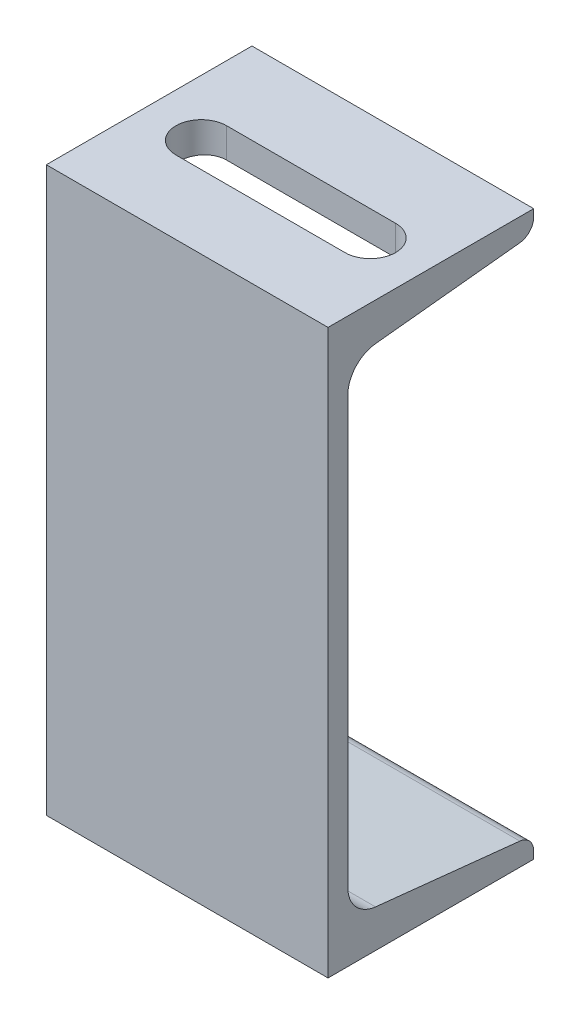
from build123d import *

# Parameters (mm, degrees)
C_20A_1_DEPTH       = 100
CUT_EXTRUDE_1_DEPTH = 16


with BuildPart() as part:
    # Sketch1 → C 槽 20A(1) (new body)
    with BuildSketch(Plane(origin=(0, 0, 0), x_dir=(0, 0, -1), z_dir=(1, 0, 0))):
        with BuildLine():
            Line((73, 200), (0, 200))
            Line((0, 200), (0, 0))
            Line((0, 0), (73, 0))
            Line((73, 0), (73, 2.579337993))
            ThreePointArc((73, 2.579337993), (71.58729654, 6.259556328), (68.074906548, 8.049208417))
            Line((68.074906548, 8.049208417), (16.850186904, 13.433143402))
            ThreePointArc((16.850186904, 13.433143402), (9.82540692, 17.012447581), (7, 24.372884251))
            Line((7, 24.372884251), (7, 175.627115749))
            ThreePointArc((7, 175.627115749), (9.82540692, 182.987552419), (16.850186904, 186.566856598))
            Line((16.850186904, 186.566856598), (68.074906548, 191.950791583))
            ThreePointArc((68.074906548, 191.950791583), (71.58729654, 193.740443672), (73, 197.420662007))
            Line((73, 197.420662007), (73, 200))
        make_face()
    extrude(amount=C_20A_1_DEPTH)

    # 草图2 → 切除-拉伸1 (cut)
    with BuildSketch(Plane(origin=(0, 200, 0), x_dir=(1, 0, 0), z_dir=(0, 1, 0))):
        with BuildLine():
            Line((20, 44), (80, 44))
            ThreePointArc((80, 44), (89, 35), (80, 26))
            Line((80, 26), (20, 26))
            ThreePointArc((20, 26), (11, 35), (20, 44))
        make_face()
    extrude(amount=-CUT_EXTRUDE_1_DEPTH, mode=Mode.SUBTRACT)


solid = part.part
